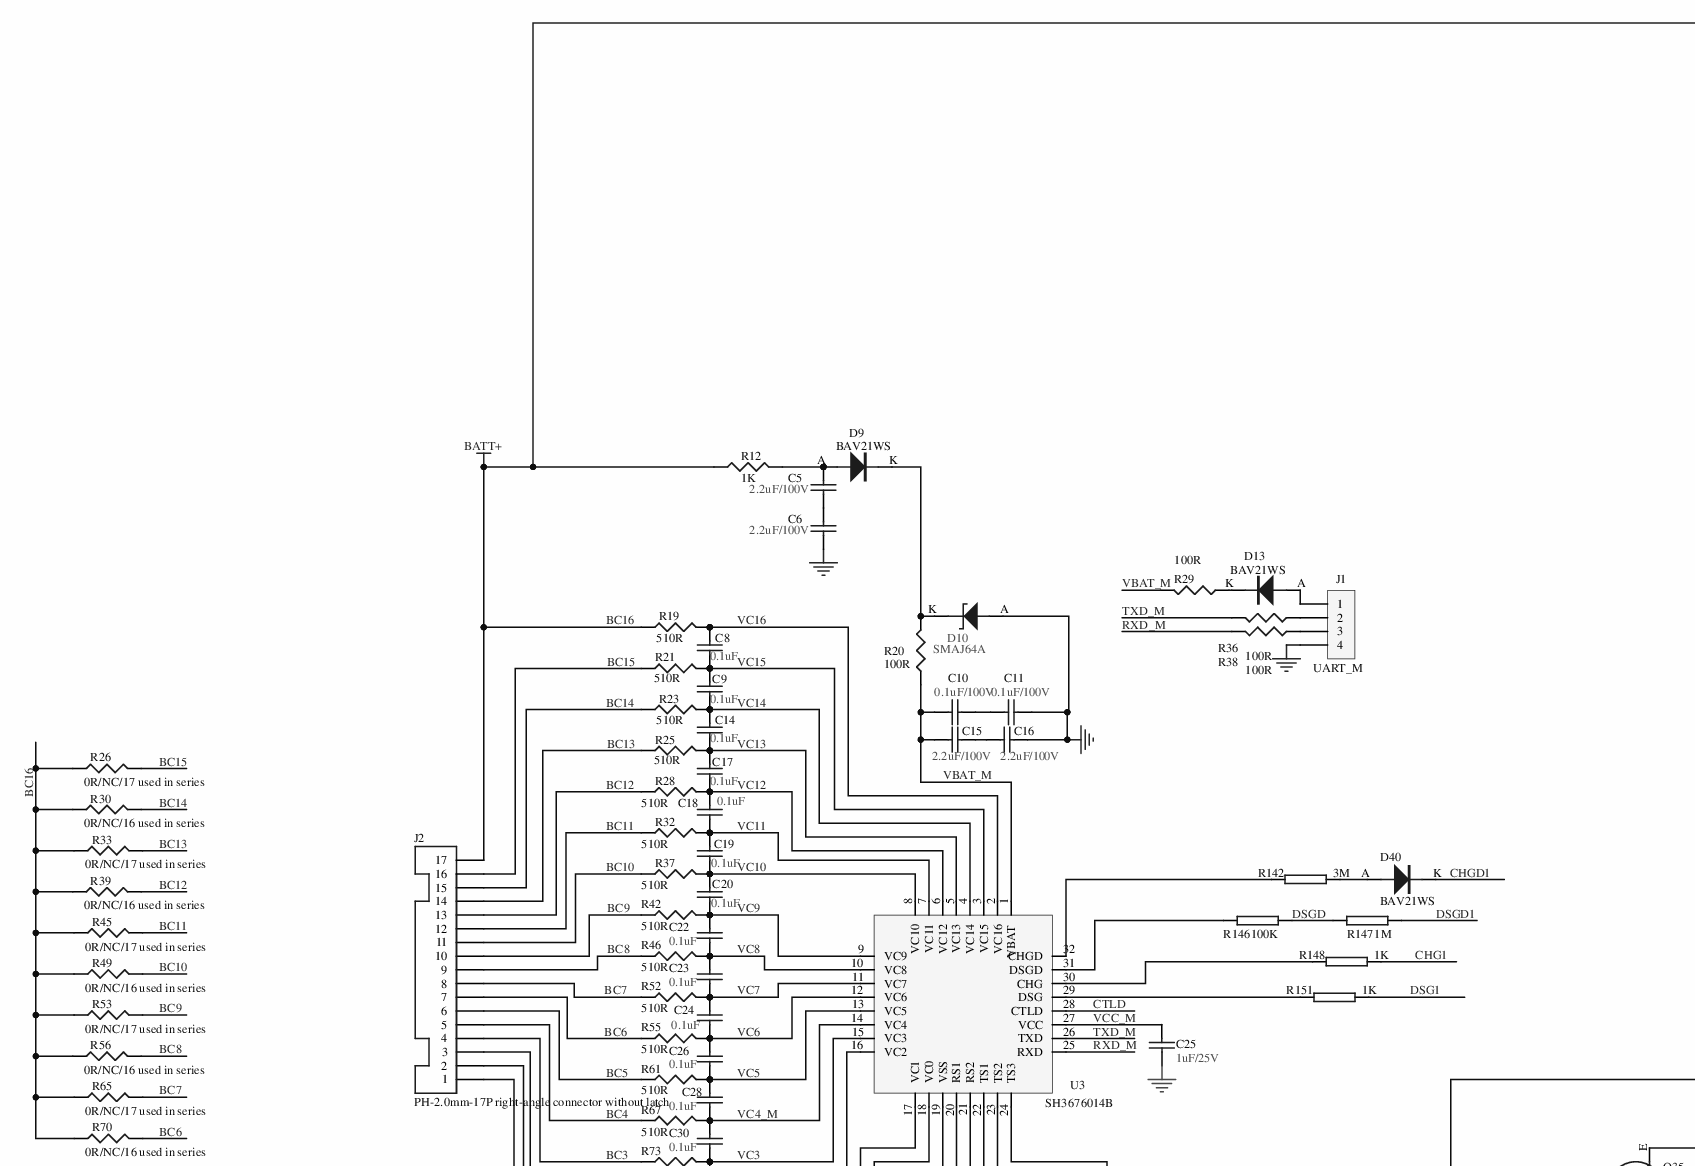
[diagram p0: MISC86327.schDOC, top left]
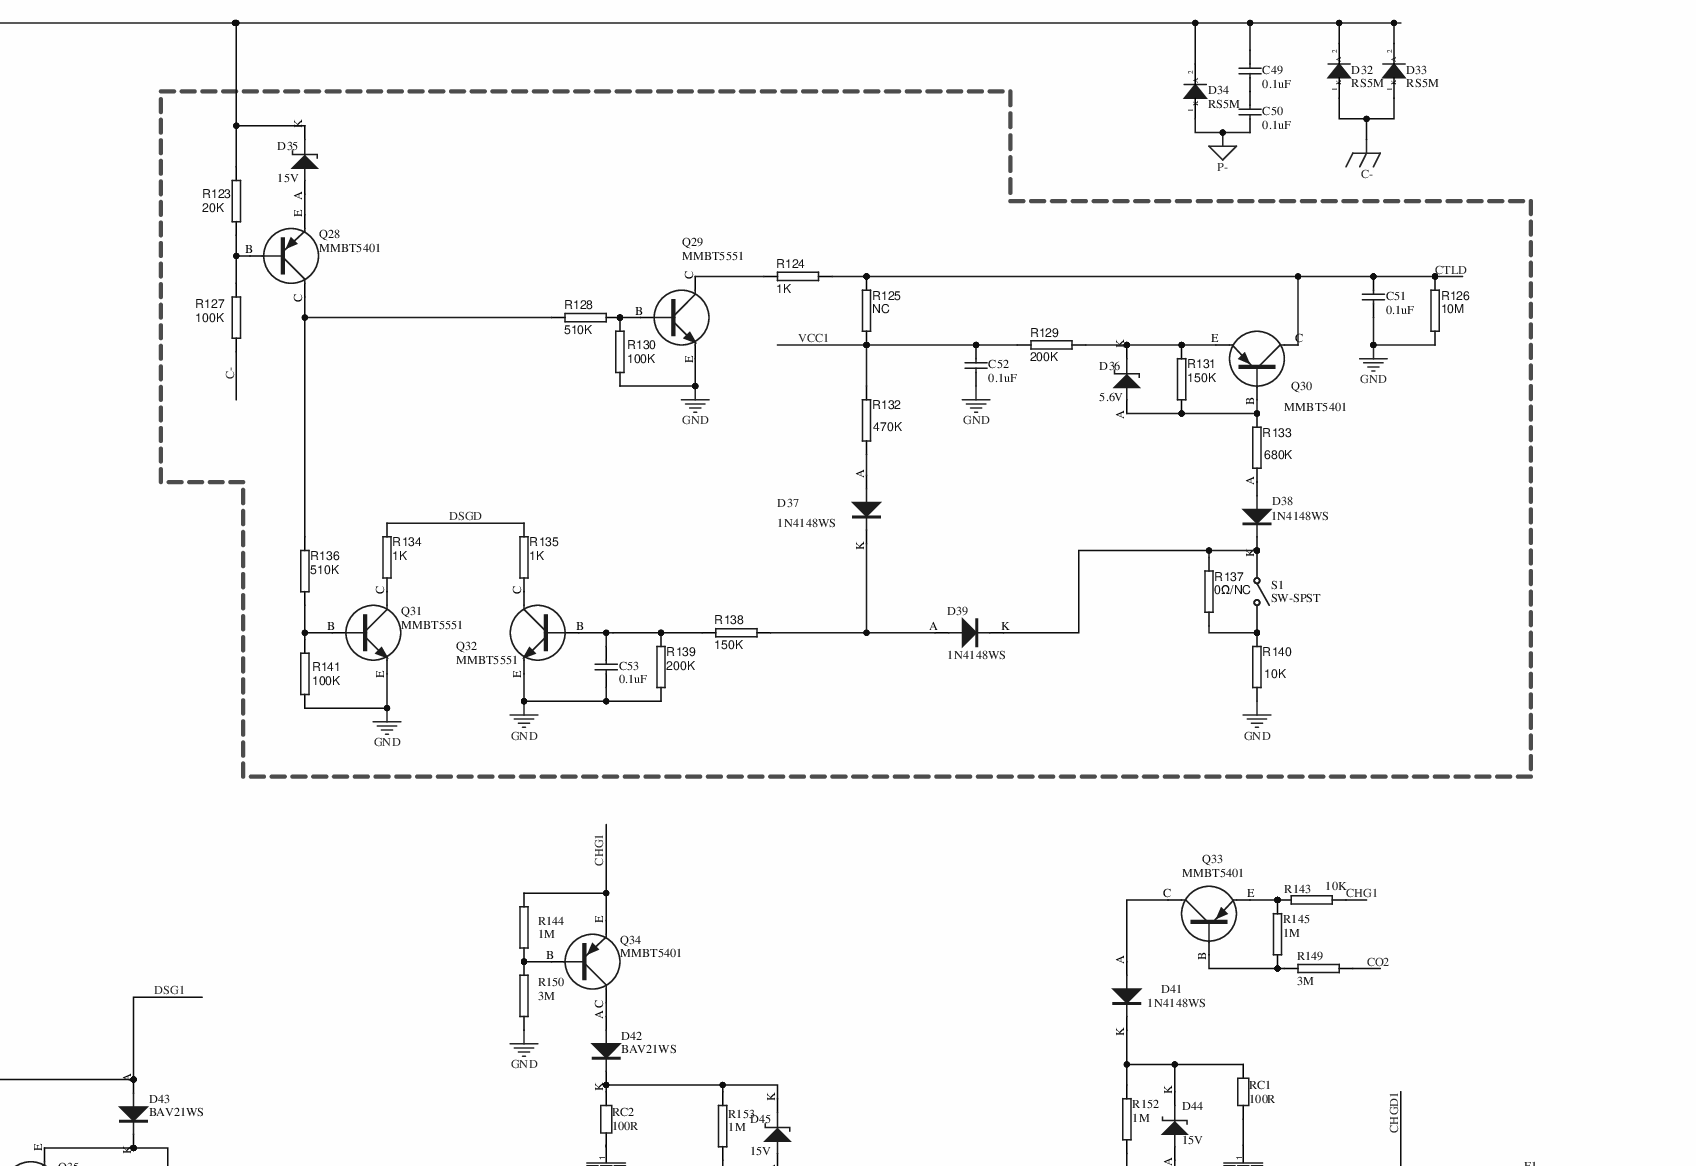
[diagram p1: MISC86327.schDOC, top right]
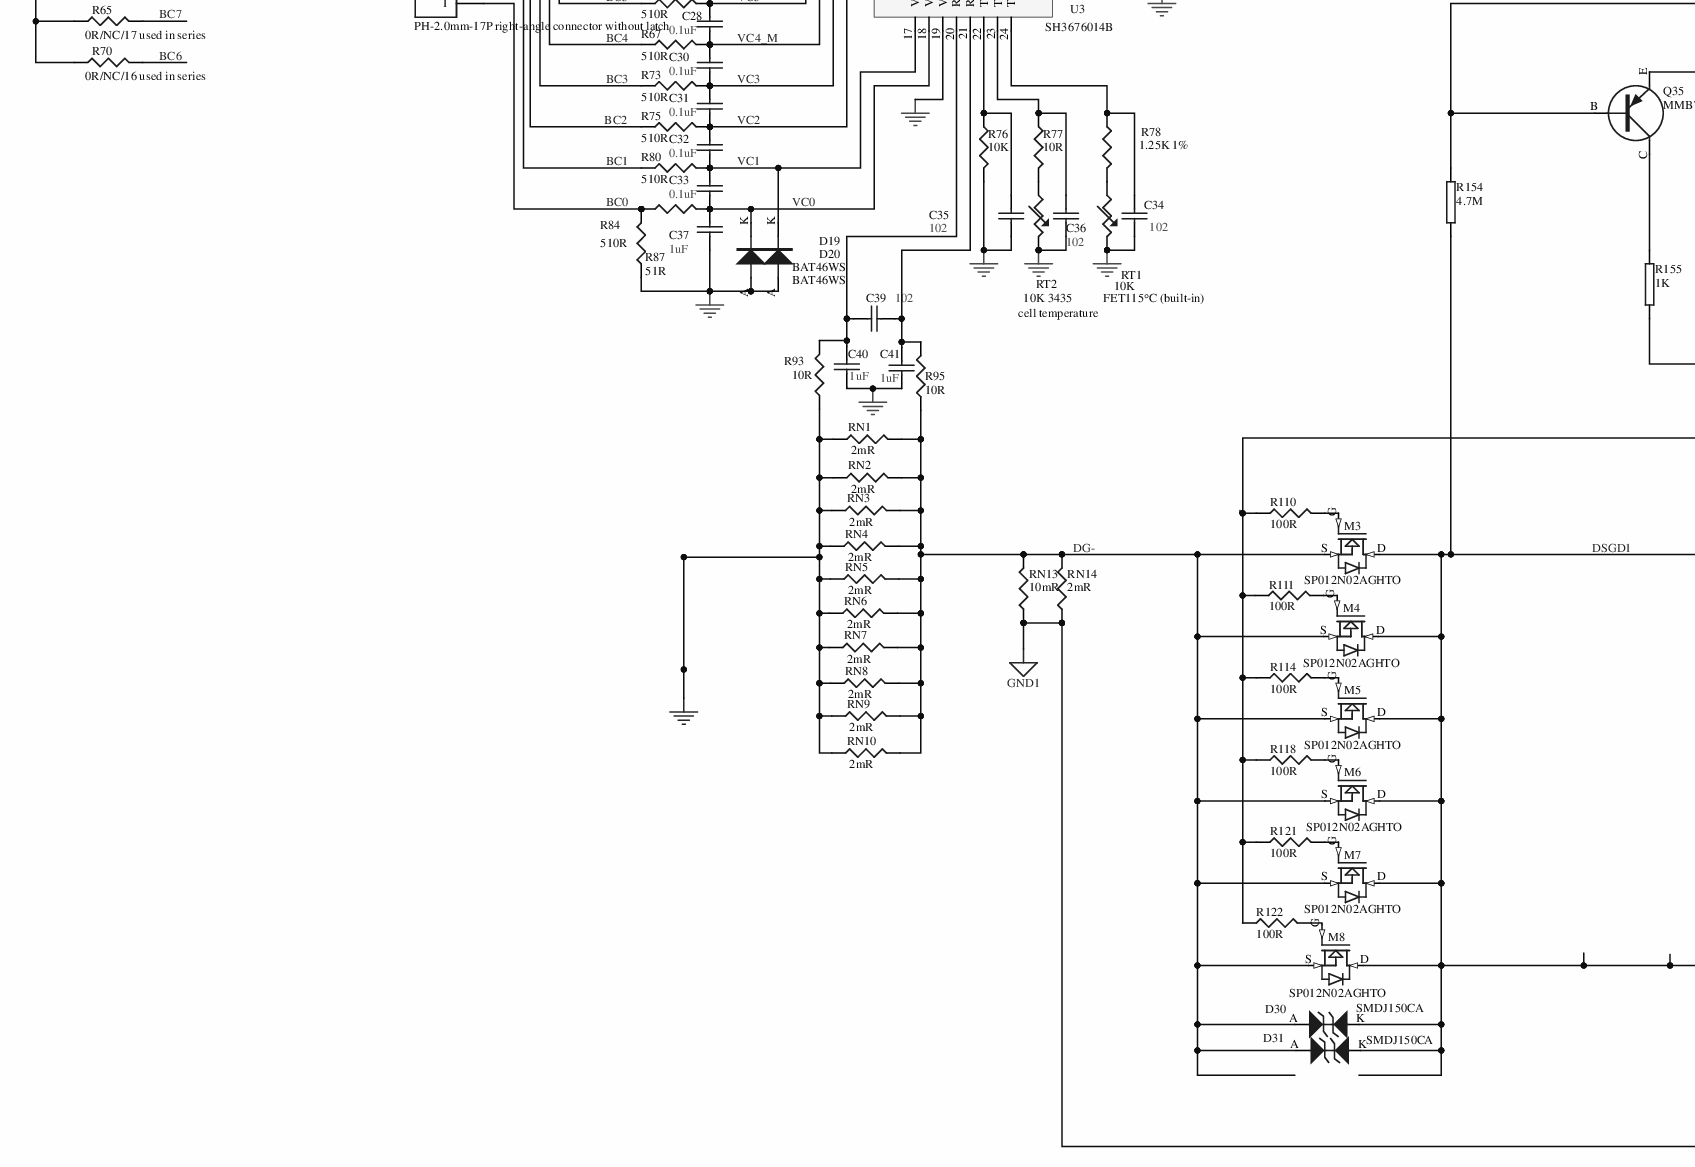
[diagram p2: MISC86327.schDOC, bottom left]
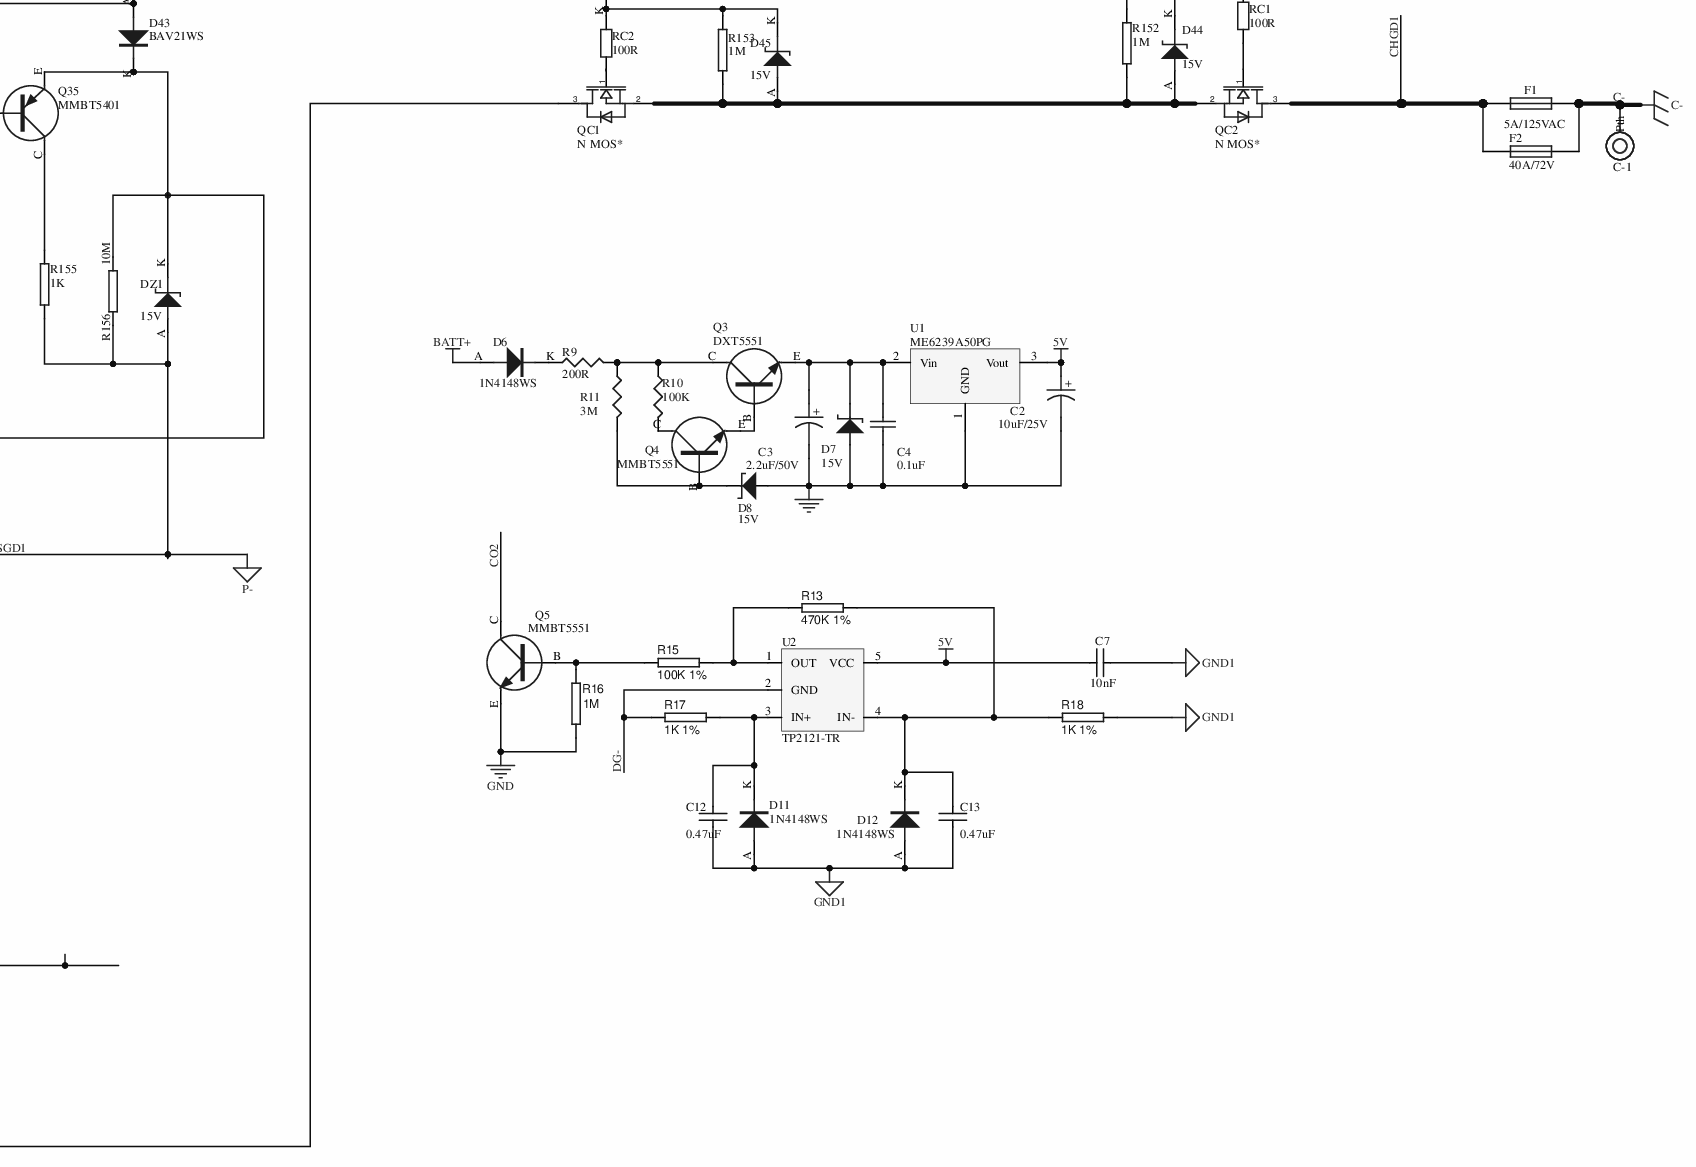
[diagram p3: MISC86327.schDOC, bottom right]
# Altium project MISC86327.PrjPcb
1 sheet, 198 parts. Net scope: global (net labels, ports and power ports of the same name join across sheets).
Board file: MISC86327.PcbDoc

## Sheet MISC86327.schDOC
size 800 x 650 mm; SheetNumber: 1; SheetTotal: 1

### Parts
C2  10uF/25V  [C0805]
C3  2.2uF/50V  [C0805]
C4  0.1uF  [C0603M]
C5  2.2uF/100V  [C0805]
C6  2.2uF/100V  [C0805]
C7  10nF  [C0603M]
C8  0.1uF  [C0603M]
C9  0.1uF  [C0603M]
C10  0.1uF/100V  [C0805]
C11  0.1uF/100V  [C0805]
C12  0.47uF  [C0603M]
C13  0.47uF  [C0603M]
C14  0.1uF  [C0603M]
C15  2.2uF/100V  [C0805]
C16  2.2uF/100V  [C0805]
C17  0.1uF  [C0603M]
C18  0.1uF  [C0603M]
C19  0.1uF  [C0603M]
C20  0.1uF  [C0603M]
C22  0.1uF  [C0603M]
C23  0.1uF  [C0603M]
C24  0.1uF  [C0603M]
C25  1uF/25V  [C0603M]
C26  0.1uF  [C0603M]
C28  0.1uF  [C0603M]
C30  0.1uF  [C0603M]
C31  0.1uF  [C0603M]
C32  0.1uF  [C0603M]
C33  0.1uF  [C0603M]
C34  102  [C0603M]
C35  102  [C0603M]
C36  102  [C0603M]
C37  1uF  [C0603M]
C39  102  [C0603M]
C40  1uF  [C0603M]
C41  1uF  [C0603M]
C49  0.1uF  [C0603A]
C50  0.1uF  [C0603A]
C51  0.1uF  [C0603A]
C52  0.1uF  [C0603A]
C53  0.1uF  [C0603A]
C-1  Pth  [4*3]
D6  1N4148WS  [SOD-323-E]
D7  15V  [SOD-323-E]
D8  15V  [SOD-323-E]
D9  BAV21WS  [SOD-323-E]
D10  SMAJ64A  [SMA]
D11  1N4148WS  [SOD-323-E]
D12  1N4148WS  [SOD-323-E]
D13  BAV21WS  [SOD-323-E]
D19  BAT46WS  [SOD-323-E]
D20  BAT46WS  [SOD-323-E]
D30  SMDJ150CA  [SMC-BI]
D31  SMDJ150CA  [SMC-BI]
D32  RS5M  [SMC_MDO-214AB)]
D33  RS5M  [SMC_MDO-214AB)]
D34  RS5M  [SMC_MDO-214AB)]
D35  15V  [SOD323(A+K-)]
D36  5.6V  [SOD323(A+K-)]
D37  1N4148WS  [SOD323(A+K-)]
D38  1N4148WS  [SOD323(A+K-)]
D39  1N4148WS  [SOD323(A+K-)]
D40  BAV21WS  [SOD323(A+K-)]
D41  1N4148WS  [SOD323(A+K-)]
D42  BAV21WS  [SOD323(A+K-)]
D43  BAV21WS  [SOD323(A+K-)]
D44  15V  [SOD323(A+K-)]
D45  15V  [SOD323(A+K-)]
DZ1  15V  [SOD323(A+K-)]
F1  5A/125VAC  [R1206L]
F2  40A/72V  [R1206L]
J1  UART_M  [CON4/2.0]
J2  PH-2.0mm-17P right-angle connector without latch  [HY2.0WT-17A/P 卧贴带扣耐温260℃]
M3  SP012N02AGHTO  [TOLL]
M4  SP012N02AGHTO  [TOLL]
M5  SP012N02AGHTO  [TOLL]
M6  SP012N02AGHTO  [TOLL]
M7  SP012N02AGHTO  [TOLL]
M8  SP012N02AGHTO  [TOLL]
Q3  DXT5551  [SOT-89BCE]
Q4  MMBT5551  [SOT-23S]
Q5  MMBT5551  [SOT-23S]
Q28  MMBT5401  [SOT23-3_BEC]
Q29  MMBT5551  [SOT23-3_BEC]
Q30  MMBT5401  [SOT23-3_BEC]
Q31  MMBT5551  [SOT23-3_BEC]
Q32  MMBT5551  [SOT23-3_BEC]
Q33  MMBT5401  [SOT23-3_BEC]
Q34  MMBT5401  [SOT23-3_BEC]
Q35  MMBT5401  [SOT23-3_BEC]
QC1  N MOS*  [TOLL]
QC2  N MOS*  [TOLL]
R9  200R  [R0805]
R10  100K  [R0603m]
R11  3M  [R0603m]
R12  1K  [R0805]
R13  470K 1%  [R0603m]
R15  100K 1%  [R0603m]
R16  1M  [R0603m]
R17  1K 1%  [R0603m]
R18  1K 1%  [R0603m]
R19  510R  [R0603m]
R20  100R  [R0805]
R21  510R  [R0603m]
R23  510R  [R0603m]
R25  510R  [R0603m]
R26  0R/NC/17 used in series  [R0805A]
R28  510R  [R0603m]
R29  100R  [R0603m]
R30  0R/NC/16 used in series  [R0805A]
R32  510R  [R0603m]
R33  0R/NC/17 used in series  [R0805A]
R36  100R  [R0603m]
R37  510R  [R0603m]
R38  100R  [R0603m]
R39  0R/NC/16 used in series  [R0805A]
R42  510R  [R0603m]
R45  0R/NC/17 used in series  [R0805A]
R46  510R  [R0603m]
R49  0R/NC/16 used in series  [R0805A]
R52  510R  [R0603m]
R53  0R/NC/17 used in series  [R0805A]
R55  510R  [R0603m]
R56  0R/NC/16 used in series  [R0805A]
R61  510R  [R0603m]
R65  0R/NC/17 used in series  [R0805A]
R67  510R  [R0603m]
R70  0R/NC/16 used in series  [R0805A]
R73  510R  [R0603m]
R75  510R  [R0603m]
R76  10K  [R0603m]
R77  10R  [R0603m]
R78  1.25K 1%  [R0603m]
R80  510R  [R0603m]
R84  510R  [R0603m]
R87  51R  [R0805]
R93  10R  [R0603m]
R95  10R  [R0603m]
R110  100R  [R0603m]
R111  100R  [R0603m]
R114  100R  [R0603m]
R118  100R  [R0603m]
R121  100R  [R0603m]
R122  100R  [R0603m]
R123  20K  [R0603A]
R124  1K  [R0603A]
R125  NC  [R0603A]
R126  10M  [R0603A]
R127  100K  [R0603A]
R128  510K  [R0603A]
R129  200K  [R0603A]
R130  100K  [R0603A]
R131  150K  [R0603A]
R132  470K  [R0603A]
R133  680K  [R0603A]
R134  1K  [R0603A]
R135  1K  [R0603A]
R136  510K  [R0603A]
R137  0Ω/NC  [R0603A]
R138  150K  [R0603A]
R139  200K  [R0603A]
R140  10K  [R0603A]
R141  100K  [R0603A]
R142  3M  [R0603A]
R143  10K  [R0603A]
R144  1M  [R0603A]
R145  1M  [R0603A]
R146  100K  [R0603A]
R147  1M  [R0603A]
R148  1K  [R0603A]
R149  3M  [R0603A]
R150  3M  [R0603A]
R151  1K  [R0603A]
R152  1M  [R0603A]
R153  1M  [R0603A]
R154  4.7M  [R0603A]
R155  1K  [R0603A]
R156  10M  [R0603A]
RC1  100R  [R0603A]
RC2  100R  [R0603A]
RN1  2mR  [R2512A]
RN2  2mR  [R2512A]
RN3  2mR  [R2512A]
RN4  2mR  [R2512A]
RN5  2mR  [R2512A]
RN6  2mR  [R2512A]
RN7  2mR  [R2512A]
RN8  2mR  [R2512A]
RN9  2mR  [R2512A]
RN10  2mR  [R2512A]
RN13  10mR  [R2512A]
RN14  2mR  [R2512A]
RT1  10K  [R0603]
RT2  10K 3435  [NTC-DIP]
S1  SW-SPST  [NTC-DIP]
U1  ME6239A50PG  [SO-89]
U2  TP2121-TR  [SOT23-5]
U3  SH3676014B  [LQFP-32]

### Nets
5V: C2.1 C7.1 U1.3(Vout) U2.5(VCC)
BC16: C49.2 D6.A D32.2(A) D33.2(A) D34.2(A) D35.K J2.17 R12.1 R19.1 R26.1 R30.1 R33.1 R39.1 R45.1 R49.1 R53.1 R56.1 R65.1 R70.1 R123.2  [also labelled BATT+]
C-: C-1.1 D32.1(K) D33.1(K) F1.2 F2.2 R127.1
DSGD1: C50.1 D30.K D31.K D34.1(K) DZ1.A M3.D M4.D M5.D M6.D M7.D M8.D R147.1 R154.1 R155.2 R156.1  [also labelled P-]
GND: C2.2 C3.2 C4.2 C6.1 C11.2 C16.2 C25.2 C34.1 C35.1 C36.1 C37.2 C40.2 C41.2 C51.1 C52.1 C53.1 D7.A D8.A D10.A D19.A D20.A J1.4 Q5.E Q29.E Q31.E Q32.E R16.1 R76.2 R87.1 R93.1 R126.1 R130.1 R139.1 R140.2 R141.1 R150.2 RN1.1 RN2.1 RN3.1 RN4.1 RN5.1 RN6.1 RN7.1 RN8.1 RN9.1 RN10.1 RT1.2 RT2.2 U1.1(GND) U3.19(VSS)
GND1: C7.2 C12.2 C13.2 D11.A D12.A QC1.3(D) R18.1 RN13.1 RN14.1
BC0: J2.1 R84.1 R87.2
BC1: J2.2 R80.1
BC2: J2.3 R75.1
BC3: J2.4 R73.1
BC4: J2.5 R67.1
BC5: J2.6 R61.1
BC6: J2.7 R55.1 R70.2
BC7: J2.8 R52.1 R65.2
BC8: J2.9 R46.1 R56.2
BC9: J2.10 R42.1 R53.2
BC10: J2.11 R37.1 R49.2
BC11: J2.12 R32.1 R45.2
BC12: J2.13 R28.1 R39.2
BC13: J2.14 R25.1 R33.2
BC14: J2.15 R23.1 R30.2
BC15: J2.16 R21.1 R26.2
CHG1: Q34.E R143.2 R144.2 R148.1
CHGD1: D40.K F1.1 F2.1 QC2.3(D)
CO2: Q5.C R149.1
CTLD: C51.2 Q30.C R124.2 R125.1 R126.2 U3.28(CTLD)
DG-: D30.A D31.A M3.S M4.S M5.S M6.S M7.S M8.S R17.2 R95.1 RN1.2 RN2.2 RN3.2 RN4.2 RN5.2 RN6.2 RN7.2 RN8.2 RN9.2 RN10.2 RN13.2 RN14.2 U2.2(GND)
DSG1: D43.A Q35.B R151.1 R154.2
DSGD: R134.2 R135.2 R146.1 R147.2
RXD_M: R36.2 U3.25(RXD)
TXD_M: R38.2 U3.26(TXD)
VBAT_M: C10.1 C15.1 R20.1 R29.2 U3.1(VBAT)
VC0: C33.2 C37.1 D20.K R84.2 U3.18(VC0)
VC1: C32.2 C33.1 D19.K R80.2 U3.17(VC1)
VC2: C31.2 C32.1 R75.2 U3.16(VC2)
VC3: C30.2 C31.1 R73.2 U3.15(VC3)
VC4_M: C28.2 C30.1 R67.2 U3.14(VC4)
VC5: C26.2 C28.1 R61.2 U3.13(VC5)
VC6: C24.2 C26.1 R55.2 U3.12(VC6)
VC7: C23.2 C24.1 R52.2 U3.11(VC7)
VC8: C22.2 C23.1 R46.2 U3.10(VC8)
VC9: C20.2 C22.1 R42.2 U3.9(VC9)
VC10: C19.2 C20.1 R37.2 U3.8(VC10)
VC11: C18.2 C19.1 R32.2 U3.7(VC11)
VC12: C17.2 C18.1 R28.2 U3.6(VC12)
VC13: C14.2 C17.1 R25.2 U3.5(VC13)
VC14: C9.2 C14.1 R23.2 U3.4(VC14)
VC15: C8.2 C9.1 R21.2 U3.3(VC15)
VC16: C8.1 R19.2 U3.2(VC16)
VCC1: C52.2 R125.2 R129.2 R132.1
VCC_M: C25.1 U3.27(VCC)
NetC3_1: C3.1 C4.1 D7.K Q3.E U1.2(Vin)
NetC5_1: C5.1 C6.2
NetC5_2: C5.2 D9.A R12.2
NetC10_2: C10.2 C11.1
NetC12_1: C12.1 D11.K R17.1 U2.3(IN+)
NetC13_1: C13.1 D12.K R13.1 R18.2 U2.4(IN-)
NetC15_2: C15.2 C16.1
NetC34_2: C34.2 R78.1 U3.24(TS3)
NetC35_2: C35.2 R76.1 U3.22(TS1)
NetC36_2: C36.2 R77.1 U3.23(TS2)
NetC39_1: C39.1 C41.1 R95.2 U3.21(RS2)
NetC39_2: C39.2 C40.1 R93.2 U3.20(RS1)
NetC49_1: C49.1 C50.2
NetC53_2: C53.2 Q32.B R138.1 R139.2
NetD6_K: D6.K R9.2
NetD8_K: D8.K Q4.B R11.2
NetD9_K: D9.K D10.K R20.2
NetD13_A: D13.A J1.1
NetD13_K: D13.K R29.1
NetD35_A: D35.A Q28.E
NetD36_A: D36.A Q30.B R131.1 R133.1
NetD36_K: D36.K Q30.E R129.1 R131.2
NetD37_A: D37.A R132.2
NetD37_K: D37.K D39.A R138.2
NetD38_A: D38.A R133.2
NetD38_K: D38.K D39.K R137.1 S1.1(COMMON)
NetD40_A: D40.A R142.1
NetD41_A: D41.A Q33.C
NetD41_K: D41.K D44.K R152.1 RC1.1
NetD42_A: D42.A Q34.C
NetD42_K: D42.K D45.K R153.2 RC2.2
NetD43_K: D43.K DZ1.K Q35.E R110.1 R111.1 R114.1 R118.1 R121.1 R122.1 R156.2
NetD44_A: D44.A D45.A QC1.2(S) QC2.2(S) R152.2 R153.1
NetJ1_2: J1.2 R38.1
NetJ1_3: J1.3 R36.1
NetM3_G: M3.G R110.2
NetM4_G: M4.G R111.2
NetM5_G: M5.G R114.2
NetM6_G: M6.G R118.2
NetM7_G: M7.G R121.2
NetM8_G: M8.G R122.2
NetQ3_B: Q3.B Q4.E
NetQ3_C: Q3.C R9.1 R10.1 R11.1
NetQ4_C: Q4.C R10.2
NetQ5_B: Q5.B R15.2 R16.2
NetQ28_B: Q28.B R123.1 R127.2
NetQ28_C: Q28.C R128.2 R136.2
NetQ29_B: Q29.B R128.1 R130.2
NetQ29_C: Q29.C R124.1
NetQ31_B: Q31.B R136.1 R141.2
NetQ31_C: Q31.C R134.1
NetQ32_C: Q32.C R135.1
NetQ33_B: Q33.B R145.1 R149.2
NetQ33_E: Q33.E R143.1 R145.2
NetQ34_B: Q34.B R144.1 R150.1
NetQ35_C: Q35.C R155.1
NetQC1_1: QC1.1(G) RC2.1
NetQC2_1: QC2.1(G) RC1.2
NetR13_2: R13.2 R15.1 U2.1(OUT)
NetR77_2: R77.2 RT2.1
NetR78_2: R78.2 RT1.1
NetR137_2: R137.2 R140.1 S1.2(NO)
NetR142_2: R142.2 U3.32(CHGD)
NetR146_2: R146.2 U3.31(DSGD)
NetR148_2: R148.2 U3.30(CHG)
NetR151_2: R151.2 U3.29(DSG)

### Notes on the sheet
- cell temperature
- FET115°C (built-in)

### Library data of the parts
C2 C3 = CAPACITOR POL: Capacitor
C4-C6 C8-C11 C14-C20 C22-C26 C28 C30-C37 C39-C41 = CAP: Capacitor
C7 C12 C13 = CAP
C49-C53 = 0805 100nF(104) 10% 50V: chip capacitor; ComponentLink1Description: supplier link; Package: 0805; Supplier: LC; SuppliersPartNumber: C49678
C-1 = Pth: through-hole pad
D6 D9 D11-D13 D19 D20 D37-D43 = DIODE
D7 D8 D10 D35 D36 D44 D45 DZ1 = ZENER2: Zener Diode
D30 D31 = diode-esd: bidirectional ESD
D32-D34 = RS5M: chip diode
F1 F2 = FUSE1: Fuse
J1 = CON4: Connector
J2 = PH-2.0mm-17P弯脚不带扣
M3-M8 = MOSFET N
Q3-Q5 Q29 Q31 Q32 = NPN: NPN Transistor
Q28 Q30 Q33-Q35 = PNP: PNP Transistor
QC1 QC2 = N MOS*: chip MOS
R9-R12 R19-R21 R23 R25 R26 R28-R30 R32 R33 R36-R39 R42 R45 R46 R49 R52 R53 R55 R56 R61 R65 R67 R70 R73 R75-R78 R80 R84 R87 R93 R95 R110 R111 R114 R118 R121 R122 RN1-RN10 RN13 RN14 = RES1
R13 R15-R18 R123-R142 R144 R146-R148 R150 R151 R153-R156 = RES1: RES
R143 R145 R149 R152 = RES
RC1 RC2 = 0603 1.2MΩ (1204) 1%: chip resistor; ComponentLink1Description: supplier link; Package: 0603; Supplier: LC; SuppliersPartNumber: C22766
RT1 RT2 = RES3
S1 = SW-SPST: Single-Pole, Single-Throw Switch; Published: 24-Mar-1999; LatestRevisionDate: 17-Jul-2002; LatestRevisionNote: Re-released for DXP Platform.; PackageReference: SPST-2; PackageDescription: Switch; 2 Leads; Publisher: Altium Limited
U1 = VOLTREG
U2 = TP2121-TR: S8211D
U3 = SH3676016B